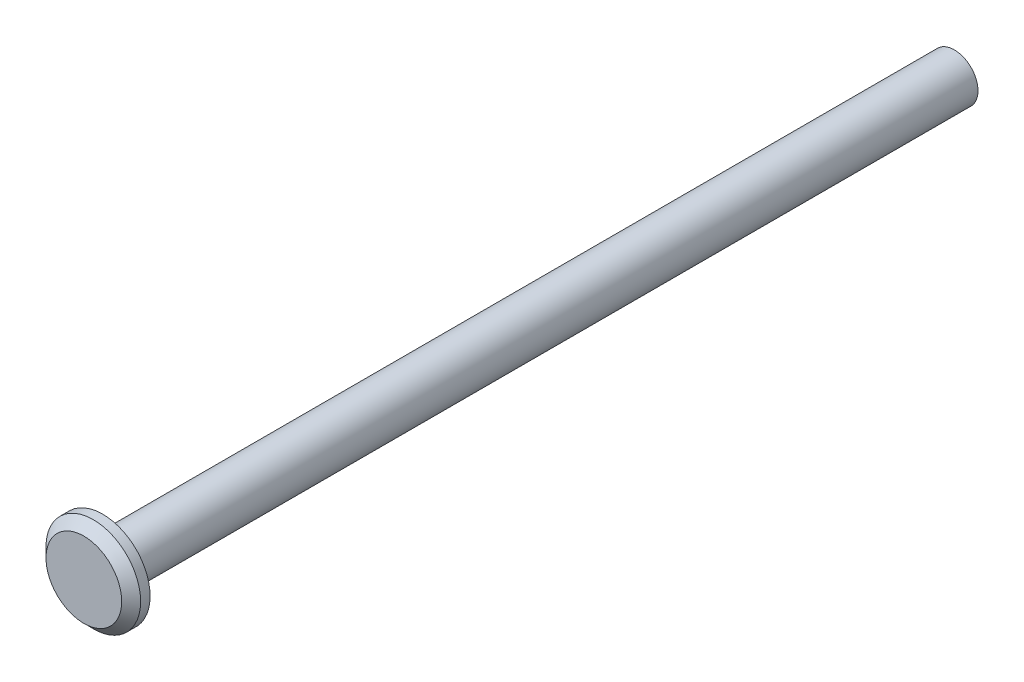
from build123d import *

# Parameters (mm, degrees)
BOSS_EXTRUDE1_DEPTH      = 2
BOSS_EXTRUDE1_DEPTH_BACK = 90
SKETCH1_R                = 2.5
SKETCH2_R                = 5
BOSS_EXTRUDE2_DEPTH      = 2
CHAMFER1_SIZE            = 1


with BuildPart() as part:
    # Sketch1 → Boss-Extrude1 (new, two sides: drawn at the far end of the back side and taken through both)
    with BuildSketch(Plane.XY.offset(-BOSS_EXTRUDE1_DEPTH_BACK)):
        Circle(SKETCH1_R)
    extrude(amount=BOSS_EXTRUDE1_DEPTH + BOSS_EXTRUDE1_DEPTH_BACK)

    # Sketch2 → Boss-Extrude2 (add)
    with BuildSketch(Plane.XY.offset(2)):
        Circle(SKETCH2_R)
    extrude(amount=-BOSS_EXTRUDE2_DEPTH)

    # Chamfer1
    chamfer1_edges = [part.edges().sort_by_distance(p)[0] for p in [
        (-5, 0, 2),
    ]]
    chamfer(chamfer1_edges, length=CHAMFER1_SIZE)


solid = part.part
